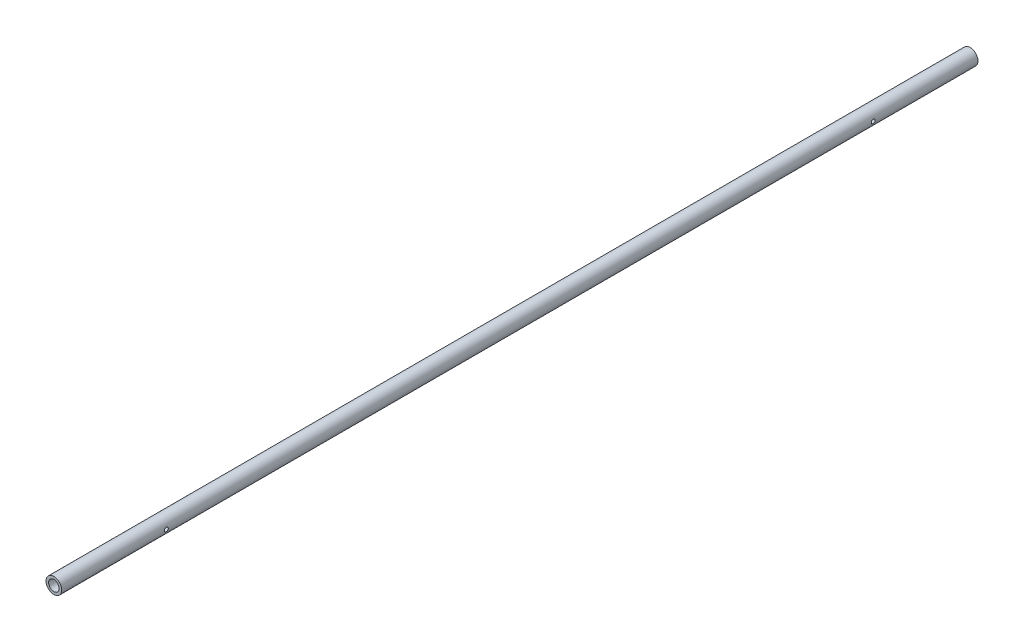
from build123d import *

# Parameters (mm, degrees)
SKETCH1_R               = 3
SKETCH1_R_2             = 2
BOSS_EXTRUDE1_DEPTH     = 350
CUT_EXTRUDE1_DEPTH      = 351.025713341
CUT_EXTRUDE1_DEPTH_BACK = 351.025713341
SKETCH3_R               = 0.75


with BuildPart() as part:
    # Sketch1 → Boss-Extrude1 (new body)
    with BuildSketch(Plane.XY):
        Circle(SKETCH1_R)
        Circle(SKETCH1_R_2, mode=Mode.SUBTRACT)
    extrude(amount=BOSS_EXTRUDE1_DEPTH)

    # Sketch3 → Cut-Extrude1 (cut, two sides: drawn at the far end of the back side and taken through both)
    with BuildSketch(Plane(origin=(0, 0, 0), x_dir=(0, 1, 0), z_dir=(-1, 0, 0)).offset(-CUT_EXTRUDE1_DEPTH_BACK)):
        with Locations(Location((0, -40, 0), (0, 0, 270))):
            Circle(SKETCH3_R)
        with Locations(Location((0, -310, 0), (0, 0, 270))):
            Circle(SKETCH3_R)
    extrude(amount=CUT_EXTRUDE1_DEPTH + CUT_EXTRUDE1_DEPTH_BACK, mode=Mode.SUBTRACT)


solid = part.part
